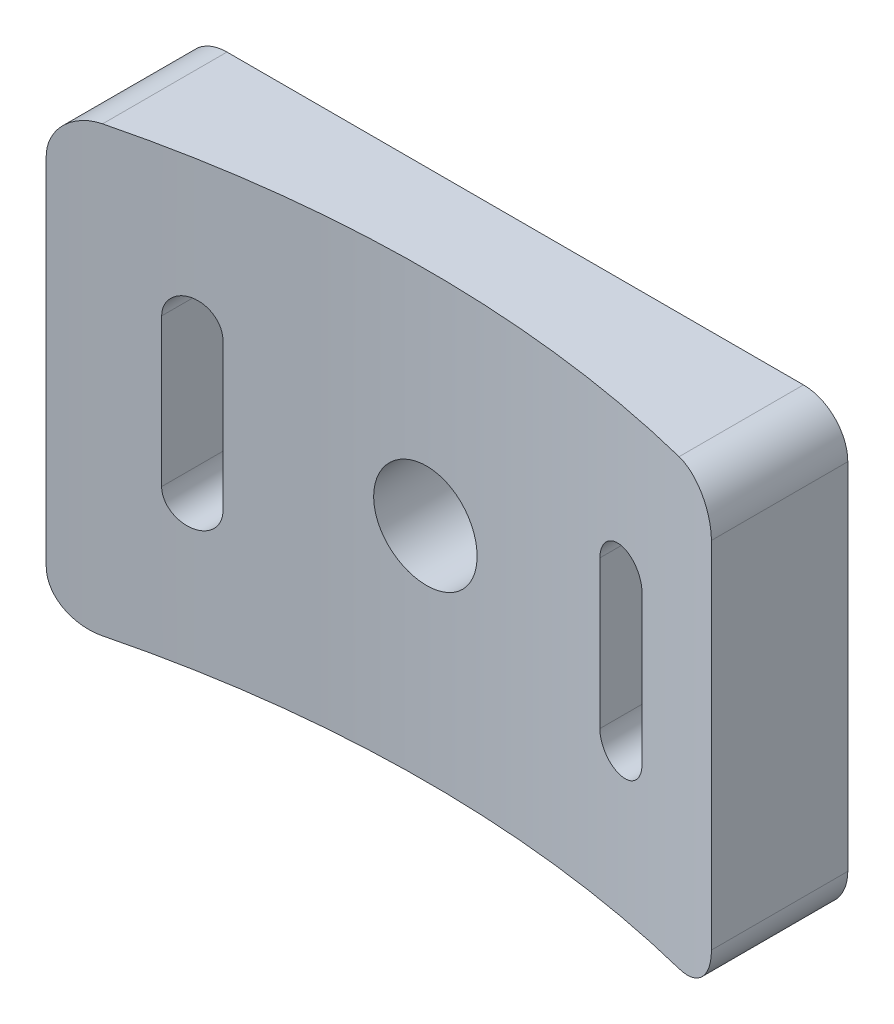
from build123d import *

# Parameters (mm, degrees)
BOSS_EXTRUDE1_DEPTH   = 30
FILLET1_R             = 3
M8X1_0_TAPPED_HOLE1_D = 7
CUT_EXTRUDE1_DEPTH    = 39.619021662
CUT_EXTRUDE2_DEPTH    = 3.3


with BuildPart() as part:
    # Sketch1 → Boss-Extrude1 (new body)
    with BuildSketch(Plane(origin=(0, 0, 0), x_dir=(1, 0, 0), z_dir=(0, 1, 0))):
        with BuildLine():
            Line((-22.5, 76.770762664), (-22.5, 86))
            Line((-22.5, 86), (22.5, 86))
            Line((22.5, 86), (22.5, 76.770762664))
            ThreePointArc((22.5, 76.770762664), (0, 80), (-22.5, 76.770762664))
        make_face()
    extrude(amount=BOSS_EXTRUDE1_DEPTH)

    # Fillet1
    fillet1_edges = [part.edges().sort_by_distance(p)[0] for p in [
        (22.5, 30, -81.385381332),
        (22.5, 0, -81.385381332),
        (-22.5, 0, -81.385381332),
        (-22.5, 30, -81.385381332),
    ]]
    fillet(fillet1_edges, radius=FILLET1_R)

    # M8x1.0 Tapped Hole1 (through all)
    with Locations(Plane(origin=(0, 0, -86), x_dir=(-1, 0, 0), z_dir=(0, 0, -1))):
        with Locations((0, 15)):
            Hole(M8X1_0_TAPPED_HOLE1_D / 2)

    # Sketch4 → Cut-Extrude1 (cut, through all)
    with BuildSketch(Plane(origin=(0, 0, -86), x_dir=(-1, 0, 0), z_dir=(0, 0, -1))):
        with BuildLine():
            Line((-12.75, 20), (-12.75, 10))
            ThreePointArc((-12.75, 10), (-14.5, 8.25), (-16.25, 10))
            Line((-16.25, 10), (-16.25, 20))
            ThreePointArc((-16.25, 20), (-14.5, 21.75), (-12.75, 20))
        make_face()
        with BuildLine():
            Line((16.25, 20), (16.25, 10))
            ThreePointArc((16.25, 10), (14.5, 8.25), (12.75, 10))
            Line((12.75, 10), (12.75, 20))
            ThreePointArc((12.75, 20), (14.5, 21.75), (16.25, 20))
        make_face()
    extrude(amount=-CUT_EXTRUDE1_DEPTH, mode=Mode.SUBTRACT)

    # Sketch5 → Cut-Extrude2 (cut)
    with BuildSketch(Plane(origin=(0, 0, -86), x_dir=(-1, 0, 0), z_dir=(0, 0, -1))):
        with BuildLine():
            Line((-11.5, 20), (-11.5, 10))
            ThreePointArc((-11.5, 10), (-14.5, 7), (-17.5, 10))
            Line((-17.5, 10), (-17.5, 20))
            ThreePointArc((-17.5, 20), (-14.5, 23), (-11.5, 20))
        make_face()
        with BuildLine():
            Line((17.5, 20), (17.5, 10))
            ThreePointArc((17.5, 10), (14.5, 7), (11.5, 10))
            Line((11.5, 10), (11.5, 20))
            ThreePointArc((11.5, 20), (14.5, 23), (17.5, 20))
        make_face()
    extrude(amount=-CUT_EXTRUDE2_DEPTH, mode=Mode.SUBTRACT)


solid = part.part
